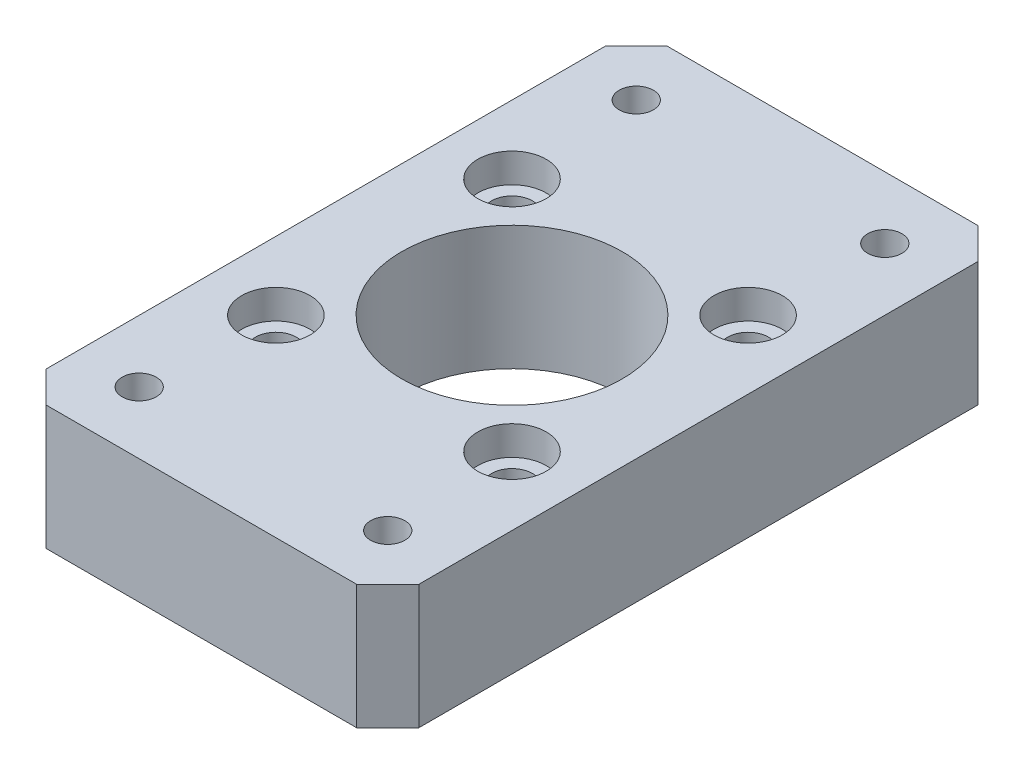
SolidWorks part; units mm, degrees
material "A6061 T6"
ref_plane "前视基准面" through (0, 0, 0) normal (0, 0, 1) x (1, 0, 0)
ref_plane "上视基准面" through (0, 0, 0) normal (0, 1, 0) x (1, 0, 0)
ref_plane "右视基准面" through (0, 0, 0) normal (1, 0, 0) x (0, 0, -1)
sketch "草图1" plane through (0, 0, 0) normal (0, 1, 0) x (1, 0, 0)
  line L1 (-30, 50) -> (30, 50)
  line L2 (-30, 50) -> (-30, -50)
  line L3 (-30, -50) -> (30, -50)
  line L4 (30, 50) -> (30, -50)
  line L5 (-30, 50) -> (30, -50) construction
  line L6 (-30, -50) -> (30, 50) construction
  point P0 (0, 0)
  dimension "D1" = 60
  dimension "D2" = 100
extrude "凸台-拉伸1" add sketch "草图1" along normal blind 20
sketch "草图2" plane through (0, 20, 0) normal (0, 1, 0) x (1, 0, 0)
  circle A0 centre (0, 0) radius 17.75
  dimension "D1" = 35.5
extrude "切除-拉伸1" cut sketch "草图2" against normal blind 20
hole_wizard "打孔尺寸(%根据)内六角花形圆柱头螺钉1" positions "草图3" profile "草图4" counterbore size "M6" standard "GB"
sketch "草图3" plane through (0, 20, 0) normal (0, 1, 0) x (1, 0, 0)
  circle A0 centre (0, 0) radius 17.75 construction
  point P0 (19, 19)
  point P2 (19, -19)
  point P4 (-19, 19)
  point P6 (-19, -19)
  dimension "D1" = 38
  dimension "D2" = 38
  dimension "D3" = 19
  dimension "D4" = 19
sketch "草图4" plane through (19, 20, -19) normal (1, 0, 0) x (0, 0, 1)
  line L0 (0, 0) -> (0, 31.9828)
  line L1 (0, 31.9828) -> (3.3, 30)
  line L2 (3.3, 30) -> (3.3, 4.7)
  line L3 (3.3, 4.7) -> (5.5, 4.7)
  line L4 (5.5, 4.7) -> (5.5, 0)
  line L5 (5.5, 0) -> (0, 0)
  line L10 (0, 31.9828) -> (-3.3, 30) construction
  line L11 (0, -6.35) -> (0, 107.95) construction
  dimension "孔直径" = 6.6
  dimension "孔深度" = 30
  dimension "柱形沉头孔直径" = 11
  dimension "柱形沉头孔深度" = 4.7
  dimension "导头角度" = 118
chamfer "倒角1" distance 5 angle 45 4 edges at (30, 10, 50) (-30, 10, 50) (-30, 10, -50) (30, 10, -50)
hole_wizard "打孔尺寸(%根据)内六角圆柱头螺钉的类型1" positions "草图5" profile "草图6" counterbore size "M5" standard "GB"
sketch "草图5" plane through (0, 0, 0) normal (0, -1, 0) x (-1, 0, 0)
  line L0 (-25, 50) -> (25, 50) construction
  line L1 (30, 45) -> (30, -45) construction
  line L2 (-30, -45) -> (-30, 45) construction
  line L3 (25, -50) -> (-25, -50) construction
  point P0 (20, 40)
  point P2 (-20, 40)
  point P4 (20, -40)
  point P6 (-20, -40)
  dimension "D1" = 10
  dimension "D2" = 10
  dimension "D3" = 10
  dimension "D4" = 10
sketch "草图6" plane through (-20, 0, -40) normal (1, 0, 0) x (0, 0, -1)
  line L0 (0, 0) -> (0, 31.6524)
  line L1 (0, 31.6524) -> (2.75, 30)
  line L2 (2.75, 30) -> (2.75, 5.7)
  line L3 (2.75, 5.7) -> (5, 5.7)
  line L4 (5, 5.7) -> (5, 0)
  line L5 (5, 0) -> (0, 0)
  line L10 (0, 31.6524) -> (-2.75, 30) construction
  line L11 (0, -6.35) -> (0, 107.95) construction
  dimension "孔直径" = 5.5
  dimension "孔深度" = 30
  dimension "柱形沉头孔直径" = 10
  dimension "柱形沉头孔深度" = 5.7
  dimension "导头角度" = 118
